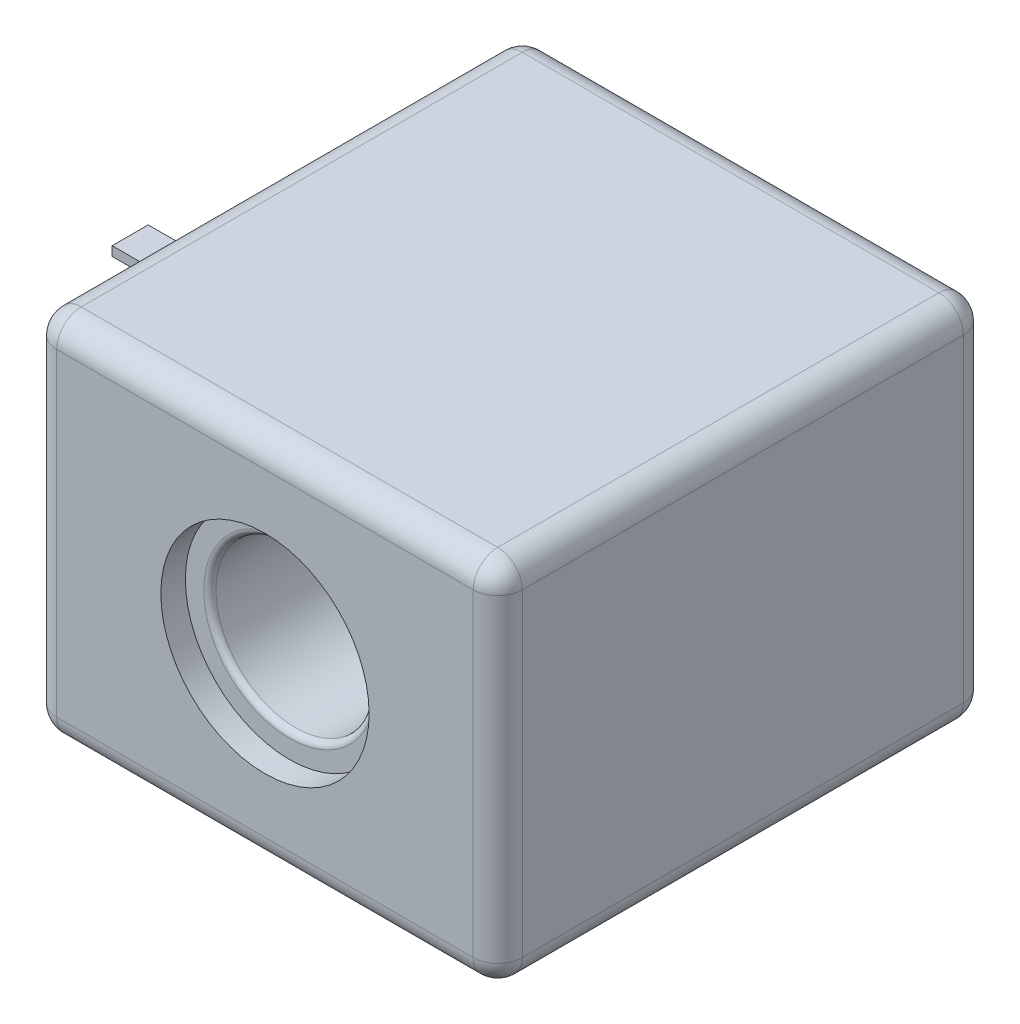
SolidWorks part; units mm, degrees
ref_plane "Front Plane" through (0, 0, 0) normal (0, 0, 1) x (1, 0, 0)
ref_plane "Top Plane" through (0, 0, 0) normal (0, 1, 0) x (1, 0, 0)
ref_plane "Right Plane" through (0, 0, 0) normal (1, 0, 0) x (0, 0, -1)
sketch "Sketch1" plane through (0, 0, 0) normal (0, 0, 1) x (1, 0, 0)
  line L1 (-19, 15) -> (19, 15)
  line L2 (-19, 15) -> (-19, -15)
  line L3 (-19, -15) -> (19, -15)
  line L4 (19, 15) -> (19, -15)
  line L5 (-19, 15) -> (19, -15) construction
  line L6 (-19, -15) -> (19, 15) construction
  point P0 (0, 0)
extrude "Boss-Extrude1" add sketch "Sketch1" along normal blind 40
fillet "Fillet1" radius 2 12 edges at (-19, -15, 20) (-19, 0, 0) (0, -15, 0) (19, -15, 20) (19, 0, 0) (19, 15, 20) (-19, 15, 20) (0, 15, 0) (0, -15, 40) (-19, 0, 40) (0, 15, 40) (19, 0, 40)
sketch "Sketch2" plane through (0, 0, 40) normal (0, 0, 1) x (1, 0, 0)
  circle A0 centre (0, 0) radius 6.5
extrude "Cut-Extrude1" cut sketch "Sketch2" against normal blind 40
sketch "Sketch3" plane through (0, 0, 40) normal (0, 0, 1) x (1, 0, 0)
  circle A0 centre (0, 0) radius 8.5
extrude "Cut-Extrude2" cut sketch "Sketch3" against normal blind 2
sketch "Sketch4" plane through (0, 0, 0) normal (0, 0, -1) x (-1, 0, 0)
  circle A0 centre (0, 0) radius 8.5
extrude "Cut-Extrude3" cut sketch "Sketch4" against normal blind 2
fillet "Fillet2" radius 0.5 2 edges at (-6.5, 0, 2) (6.5, 0, 38)
sketch "Sketch5" plane through (-19, 0, 0) normal (-1, 0, 0) x (0, 0, 1)
  circle A0 centre (20, 0) radius 1.5
extrude "Cut-Extrude4" cut sketch "Sketch5" against normal blind 9
sketch "Sketch6" plane through (-19, 0, 0) normal (-1, 0, 0) x (0, 0, 1)
  circle A0 centre (20, 0) radius 2.5
  circle A1 centre (20, 0) radius 2.499
extrude "Cut-Extrude5" cut sketch "Sketch6" against normal blind 9
sketch "Sketch7" plane through (-19, 0, 0) normal (-1, 0, 0) x (0, 0, 1)
  line L0 (21.7295, -6.2978) -> (21.5295, -6.2978)
  line L1 (24.4716, -7.0624) -> (21.5295, -7.0624)
  line L2 (24.4716, -7.0624) -> (24.4716, -6.2978)
  line L3 (24.4716, -6.2978) -> (24.2715, -6.2978)
  line L4 (21.5295, -7.0624) -> (21.5295, -6.2978)
  line L5 (24.4716, -7.0624) -> (21.5295, -6.2978) construction
  line L6 (24.4716, -6.2978) -> (21.5295, -7.0624) construction
  line L8 (24.2715, -6.2978) -> (24.2715, -6.7081)
  line L9 (24.2715, -6.7081) -> (21.7295, -6.7081)
  line L10 (21.7295, -6.2978) -> (21.7295, -6.7081)
  line L11 (22.9656, -6.2828) -> (21.7295, -6.7081) construction
  line L12 (24.2715, -6.7081) -> (22.9656, -6.2828) construction
  point P0 (23.0005, -6.6801)
  point P5 (22.9656, -6.2828)
extrude "Boss-Extrude2" add sketch "Sketch7" along normal blind 9
mirror "Mirror1" about plane through (0, 0, 0) normal (0, 1, 0) of "Boss-Extrude2"
sketch "Sketch8" plane through (-19, 0, 0) normal (-1, 0, 0) x (0, 0, 1)
  line L1 (13.5459, 1.4336) -> (14.0934, 1.4336)
  line L2 (13.5459, 1.4336) -> (13.5459, -1.4214)
  line L3 (13.5459, -1.4214) -> (14.0934, -1.4214)
  line L4 (14.0934, 1.4336) -> (14.0934, -1.4214)
  line L5 (13.5459, 1.4336) -> (14.0934, -1.4214) construction
  line L6 (13.5459, -1.4214) -> (14.0934, 1.4336) construction
  point P0 (13.8197, 0.0061)
extrude "Boss-Extrude3" add sketch "Sketch8" along normal blind 9
